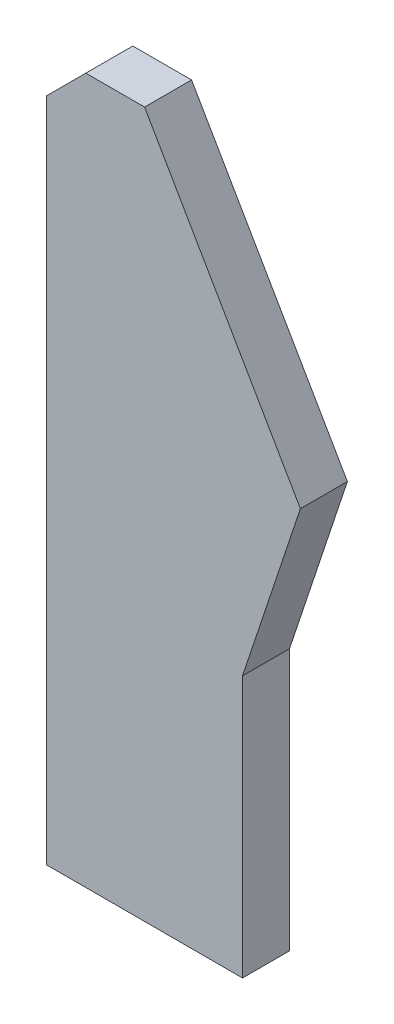
SolidWorks part; units mm, degrees
material "Q235B"
ref_plane "Front Plane" through (0, 0, 0) normal (0, 0, 1) x (1, 0, 0)
ref_plane "Top Plane" through (0, 0, 0) normal (0, 1, 0) x (1, 0, 0)
ref_plane "Right Plane" through (0, 0, 0) normal (1, 0, 0) x (0, 0, -1)
sketch "Sketch1" plane through (0, 0, 0) normal (0, 0, 1) x (1, 0, 0)
  line L0 (0, 0) -> (0, 180)
  line L1 (0, 180) -> (25, 180)
  line L2 (25, 180) -> (64.7703, 111.1158)
  line L3 (64.7703, 111.1158) -> (50, 66.792)
  line L4 (50, 66.792) -> (50, 0)
  line L5 (50, 0) -> (0, 0)
  dimension "D1" = 50
  dimension "D2" = 180
  dimension "D3" = 25
  dimension "D4" = 161.57
  dimension "D5" = 46.72
  dimension "D6" = 30
extrude "Boss-Extrude1" add sketch "Sketch1" along normal mid plane 12
chamfer "Chamfer1" distance 10 angle 45 1 edges at (0, 180, 0)
